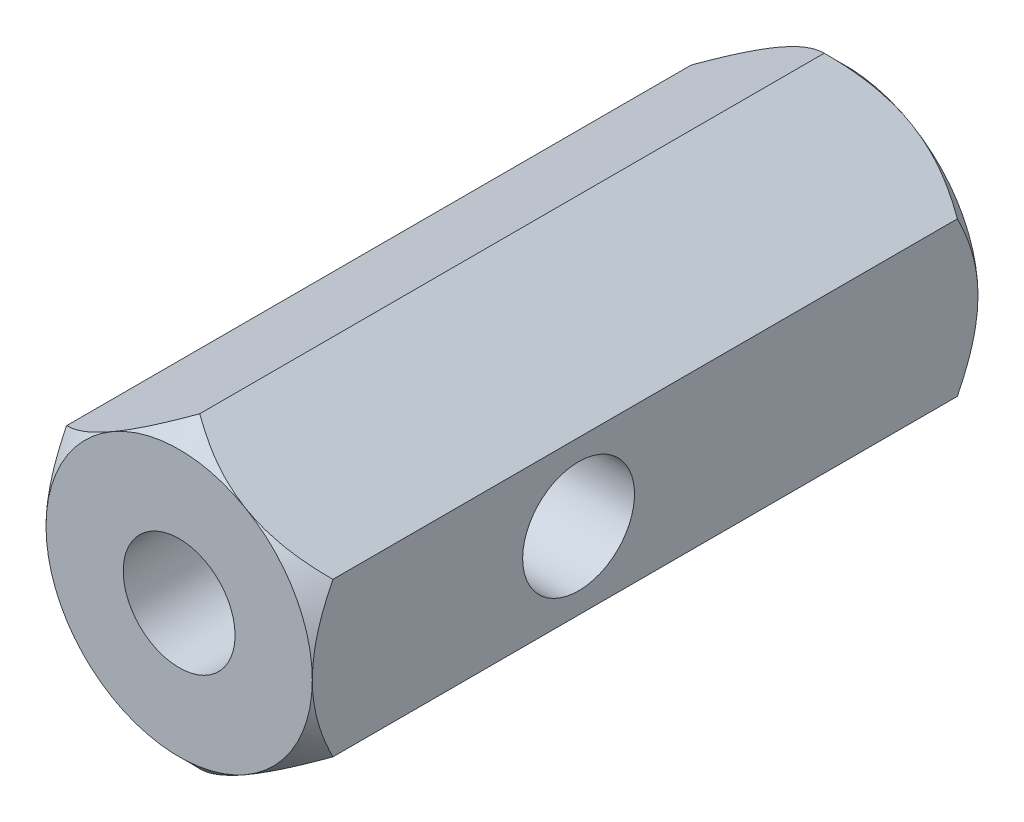
SolidWorks part; units mm, degrees
material "6063-T5"
ref_plane "Front Plane" through (0, 0, 0) normal (0, 0, 1) x (1, 0, 0)
ref_plane "Top Plane" through (0, 0, 0) normal (0, 1, 0) x (1, 0, 0)
ref_plane "Right Plane" through (0, 0, 0) normal (1, 0, 0) x (0, 0, -1)
sketch "Sketch1" plane through (0, 0, 0) normal (0, 0, 1) x (1, 0, 0)
  line L1 (0, 5.7735) -> (-5, 2.8868)
  line L2 (-5, 2.8868) -> (-5, -2.8868)
  line L3 (-5, -2.8868) -> (0, -5.7735)
  line L4 (0, -5.7735) -> (5, -2.8868)
  line L5 (5, -2.8868) -> (5, 2.8868)
  line L6 (5, 2.8868) -> (0, 5.7735)
  circle A0 centre (0, 0) radius 5 construction
  dimension "D1" = 10
extrude "Boss-Extrude1" add sketch "Sketch1" along normal blind 25
hole_wizard "M5 Tapped Hole3" positions "Sketch2" profile "Sketch3" tap size "M5" standard "ISO"
sketch "Sketch2" plane through (0, 0, 25) normal (0, 0, 1) x (1, 0, 0)
  point P0 (0, 0)
cosmetic thread "Cosmetic thread1" parameters "D1"=8, "D2"=5
sketch "Sketch3" plane through (0, 0, 25) normal (1, 0, 0) x (0, -1, 0)
  line L0 (0, 0) -> (0, 11.2618)
  line L1 (0, 11.2618) -> (2.1, 10)
  line L2 (2.1, 10) -> (2.1, 0)
  line L5 (2.1, 0) -> (0, 0)
  line L10 (0, 11.2618) -> (-2.1, 10) construction
  line L11 (0, -6.35) -> (0, 107.95) construction
  dimension "螺纹孔钻头直径" = 4.2
  dimension "螺纹孔钻头深度" = 10
  dimension "导头角度" = 118
hole_wizard "M4 Tapped Hole1" positions "Sketch4" profile "Sketch5" tap size "M4" standard "ISO"
sketch "Sketch4" plane through (0, 0, 0) normal (0, 0, -1) x (-1, 0, 0)
  point P0 (0, 0)
sketch "Sketch5" plane through (0, 0, 0) normal (1, 0, 0) x (0, 1, 0)
  line L0 (0, 0) -> (0, 9.9914)
  line L1 (0, 9.9914) -> (1.65, 9)
  line L2 (1.65, 9) -> (1.65, 0)
  line L5 (1.65, 0) -> (0, 0)
  line L10 (0, 9.9914) -> (-1.65, 9) construction
  line L11 (0, -6.35) -> (0, 107.95) construction
  dimension "螺纹孔钻头直径" = 3.3
  dimension "螺纹孔钻头深度" = 9
  dimension "导头角度" = 118
cosmetic thread "Cosmetic thread4" parameters "D1"=8, "D2"=4
hole_wizard "M5 Tapped Hole2" positions "Sketch6" profile "Sketch7" tap size "M5" standard "ISO"
sketch "Sketch6" plane through (0, 0, 0) normal (1, 0, 0) x (0, 0, -1)
  line L0 (0, -2.8868) -> (0, 2.8868) construction
  point P0 (-15, 0)
  dimension "D1" = 15
cosmetic thread "Cosmetic thread3" parameters "D2"=5
sketch "Sketch7" plane through (0, 0, 15) normal (0, 1, 0) x (0, 0, 1)
  line L0 (0, 0) -> (0, 5)
  line L1 (0, 5) -> (2.1, 5)
  line L2 (2.1, 5) -> (2.1, 0)
  line L5 (2.1, 0) -> (0, 0)
  line L11 (0, -6.35) -> (0, 107.95) construction
  dimension "通孔螺纹孔钻头直径" = 4.2
  dimension "通孔螺纹孔钻头深度" = 5
sketch "Sketch8" plane through (0, 0, 0) normal (1, 0, 0) x (0, 0, -1)
  line L0 (-25, 5) -> (-25, 5.7735)
  line L1 (-25, 2.8868) -> (-25, 5.7735) construction
  line L2 (-25, 5.7735) -> (-24.2265, 5.7735)
  line L3 (-24.2265, 5.7735) -> (-25, 5)
  line L4 (-25, 0) -> (0, 0) construction
  line L5 (-25, -2.8868) -> (-25, 2.8868) construction
  line L6 (0, 5) -> (0, 5.7735)
  line L7 (0, 2.8868) -> (0, 5.7735) construction
  line L8 (0, 5.7735) -> (-0.7735, 5.7735)
  line L9 (-0.7735, 5.7735) -> (0, 5)
  line L10 (-25, 5.7735) -> (0, 5.7735) construction
  dimension "D1" = 5
revolve "Cut-Revolve1" cut sketch "Sketch8" angle 360 about L4
sketch "Sketch9" plane through (0, 0, 0) normal (0, 1, 0) x (1, 0, 0)
  line L0 (0, -24.2265) -> (0, -0.7735) construction
  line L1 (4, -16) -> (9, -16)
  line L2 (4, -16) -> (4, -23)
  line L3 (4, -23) -> (9, -23)
  line L4 (9, -16) -> (9, -23)
  line L5 (2.5, -25) -> (5, -25) construction
  line L6 (0, 0) -> (0, -58.5772) construction
  line L7 (2.5, 0) -> (-2.5, 0) construction
  dimension "D1" = 4
  dimension "D2" = 2
  dimension "D3" = 7
  dimension "D4" = 5
revolve "Cut-Revolve2" [suppressed] cut sketch "Sketch9" angle 360 about L6
sketch "Sketch10" [suppressed] plane through (0, 0, 21) normal (0, 0, 1) x (1, 0, 0)
  circle A0 centre (0, 0) radius 5.5
  dimension "D1" = 11
extrude "Cut-Extrude1" [suppressed] cut sketch "Sketch10" along normal blind 10 flip side to cut
